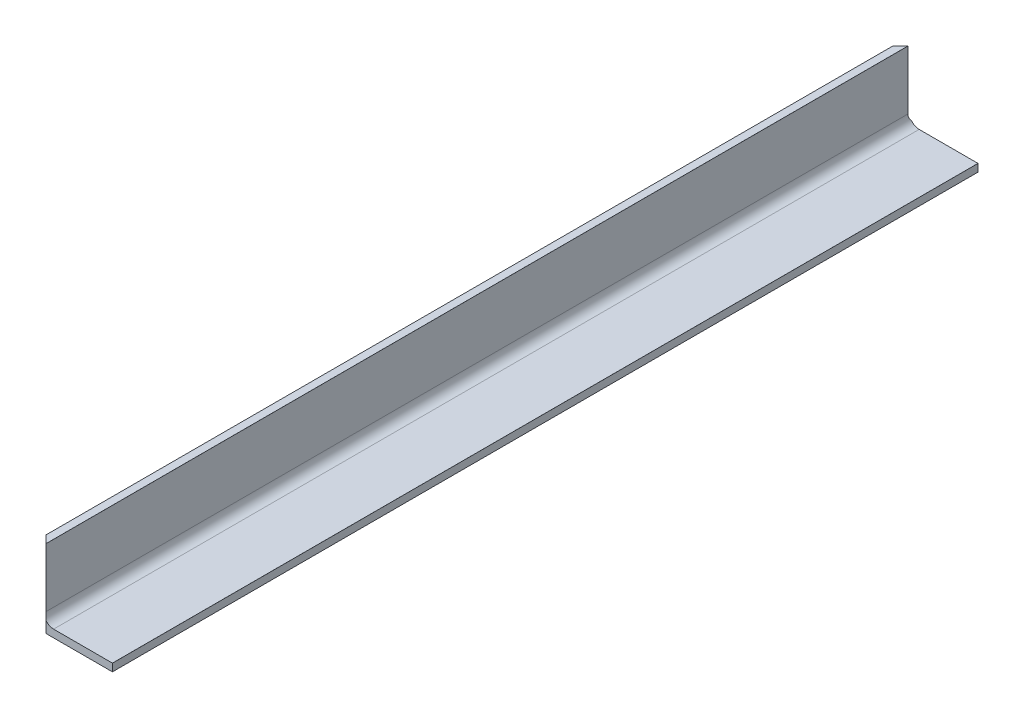
from build123d import *

# Parameters (mm, degrees)
EXTRUDE_1_DEPTH     = 456
CUT_EXTRUDE_1_DEPTH = 40


with BuildPart() as part:
    # 草图1 → 拉伸1 (new body)
    with BuildSketch(Plane.XY):
        with BuildLine():
            Line((0, 0), (0, 40))
            Line((0, 40), (3.99, 40))
            ThreePointArc((3.99, 40), (3.997071068, 39.997071068), (4, 39.99))
            Line((4, 39.99), (4, 9))
            ThreePointArc((4, 9), (5.464466094, 5.464466094), (9, 4))
            Line((9, 4), (39.99, 4))
            ThreePointArc((39.99, 4), (39.997071068, 3.997071068), (40, 3.99))
            Line((40, 3.99), (40, 0))
            Line((40, 0), (0, 0))
        make_face()
    extrude(amount=EXTRUDE_1_DEPTH)

    # 草图2 → 切除-拉伸1 (cut)
    with BuildSketch(Plane(origin=(0, 40, 0), x_dir=(1, 0, 0), z_dir=(0, 1, 0))):
        Polygon((5, -456), (0, -451), (0, -456), align=None)
        Polygon((0, 0), (0, -5), (5, 0), align=None)
    extrude(amount=-CUT_EXTRUDE_1_DEPTH, mode=Mode.SUBTRACT)


solid = part.part
